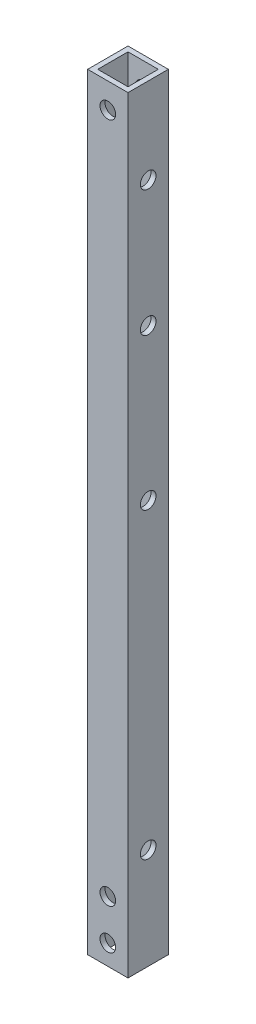
SolidWorks part; units mm, degrees
material "Thornel Mat VMA"
ref_plane "前视基准面" through (0, 0, 0) normal (0, 0, 1) x (1, 0, 0)
ref_plane "上视基准面" through (0, 0, 0) normal (0, 1, 0) x (1, 0, 0)
ref_plane "右视基准面" through (0, 0, 0) normal (1, 0, 0) x (0, 0, -1)
other "Configuration Table"
sketch "草图1" plane through (0, 0, 0) normal (0, 1, 0) x (1, 0, 0)
  line L0 (-3, 3) -> (3, 3)
  line L1 (-4, 4) -> (4, 4)
  line L2 (-4, 4) -> (-4, -4)
  line L3 (-4, -4) -> (4, -4)
  line L4 (4, 4) -> (4, -4)
  line L5 (-4, 4) -> (4, -4) construction
  line L6 (-4, -4) -> (4, 4) construction
  line L7 (3, 3) -> (3, -3)
  line L8 (-3, -3) -> (3, -3)
  line L9 (-3, 3) -> (-3, -3)
  point P0 (0, 0)
  dimension "D1" = 8
  dimension "D2" = 1
extrude "凸台-拉伸1" add sketch "草图1" along normal blind 152
sketch "草图2" plane through (0, 0, 4) normal (0, 0, 1) x (1, 0, 0)
  line L0 (4, 152) -> (4, 0) construction
  line L1 (-4, 152) -> (4, 152) construction
  line L2 (-4, 0) -> (4, 0) construction
  circle A0 centre (0, 147) radius 1.55
  circle A1 centre (0, 4) radius 1.55
  circle A2 centre (0, 12) radius 1.55
  dimension "D1" = 3.1
  dimension "D2" = 4
  dimension "D3" = 5
  dimension "D4" = 4
  dimension "D5" = 8
extrude "切除-拉伸1" cut sketch "草图2" against normal through all
sketch "草图3" plane through (4, 0, 0) normal (1, 0, 0) x (0, 0, -1)
  line L0 (-4, 152) -> (4, 152) construction
  line L1 (4, 152) -> (4, 0) construction
  circle A0 centre (0, 135) radius 1.55
  circle A1 centre (0, 20) radius 1.55
  circle A2 centre (0, 110) radius 1.55
  circle A3 centre (0, 80) radius 1.55
  dimension "D1" = 3.1
  dimension "D2" = 17
  dimension "D3" = 4
  dimension "D4" = 25
  dimension "D5" = 90
  dimension "D6" = 30
extrude "切除-拉伸2" cut sketch "草图3" against normal through all
sketch "草图5" plane through (0, 0, 4) normal (0, 0, 1) x (1, 0, 0)
  circle A0 centre (0, 147) radius 2.55
  dimension "D1" = 5.1
extrude "切除-拉伸4" [suppressed] cut sketch "草图5" against normal blind 1
sketch "草图6" plane through (4, 0, 0) normal (1, 0, 0) x (0, 0, -1)
  circle A0 centre (0, 135) radius 2.55
  dimension "D1" = 5.1
extrude "切除-拉伸5" [suppressed] cut sketch "草图6" against normal blind 1
sketch "草图7" [suppressed] plane through (0, 0, 4) normal (0, 0, 1) x (1, 0, 0)
  line L0 (0, 0) -> (0, 169.9384) construction
  line L1 (-4, 0) -> (4, 0) construction
  circle A0 centre (0, 35) radius 1.3
  circle A1 centre (0, 91) radius 1.3
  dimension "D1" = 2.6
  dimension "D2" = 56
  dimension "D3" = 35
extrude "切除-拉伸6" [suppressed] cut sketch "草图7" against normal blind 10
